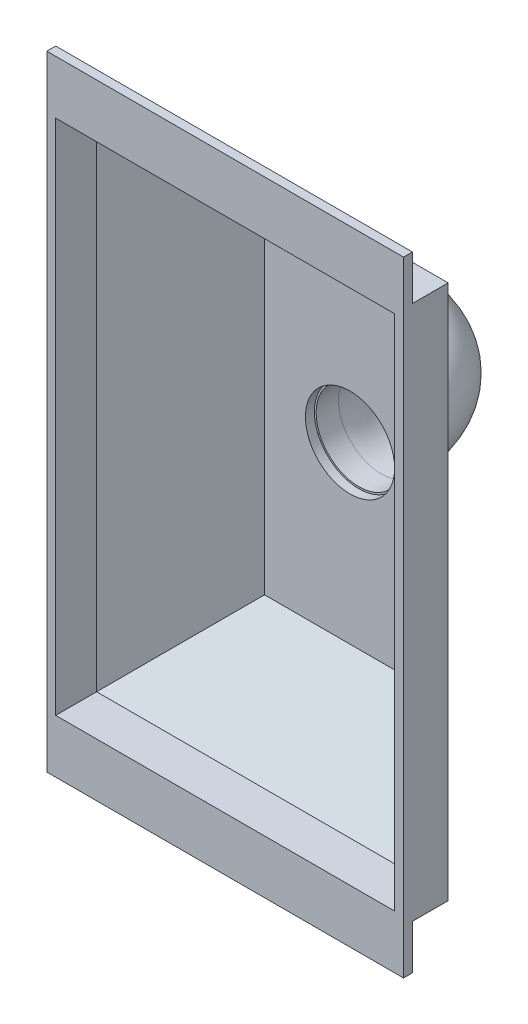
SolidWorks part; units mm, degrees
ref_plane "前视基准面" through (0, 0, 0) normal (0, 0, 1) x (1, 0, 0)
ref_plane "上视基准面" through (0, 0, 0) normal (0, 1, 0) x (1, 0, 0)
ref_plane "右视基准面" through (0, 0, 0) normal (1, 0, 0) x (0, 0, -1)
sketch "草图1" plane through (0, 0, 0) normal (0, 0, 1) x (1, 0, 0)
  line L1 (-200, -300) -> (200, -300)
  line L2 (-200, -300) -> (-200, 300)
  line L3 (-200, 300) -> (200, 300)
  line L4 (200, -300) -> (200, 300)
  line L5 (-200, -300) -> (200, 300) construction
  line L6 (-200, 300) -> (200, -300) construction
  point P0 (0, 0)
  dimension "D1" = 400
  dimension "D2" = 600
extrude "凸台-拉伸1" add sketch "草图1" along normal blind 150
sketch "草图2" plane through (0, -300, 0) normal (0, -1, 0) x (1, 0, 0)
  line L0 (0, 0) -> (0, 150) construction
  line L1 (-200, 150) -> (200, 150) construction
  line L2 (-200, 75) -> (-100, 0)
  line L3 (-200, 150) -> (-200, 0) construction
  line L4 (-200, 0) -> (200, 0) construction
  line L5 (-100, 0) -> (-200, 0)
  line L6 (-200, 0) -> (-200, 75)
  line L7 (200, 75) -> (100, 0)
  line L8 (200, 150) -> (200, 0) construction
  line L9 (100, 0) -> (200, 0)
  line L10 (200, 0) -> (200, 75)
  dimension "D1" = 200
  dimension "D2" = 100
extrude "切除-拉伸1" [suppressed] cut sketch "草图2" against normal through all
sketch "草图3" plane through (0, 0, 150) normal (0, 0, 1) x (1, 0, 0)
  line L0 (-200, -300) -> (200, -300) construction
  line L1 (-200, 300) -> (-260, 300)
  line L2 (-200, 300) -> (-200, -300)
  line L3 (-200, -300) -> (-260, -300)
  line L4 (-260, 300) -> (-260, -300)
  line L6 (200, 300) -> (260, 300)
  line L7 (200, 300) -> (200, -300)
  line L8 (200, -300) -> (260, -300)
  line L9 (260, 300) -> (260, -300)
  dimension "D1" = 60
extrude "凸台-拉伸2" [suppressed] add sketch "草图3" against normal blind 10
chamfer "倒角2" distance 100 angle 45 4 edges at (0, 300, 0) (-200, 0, 0) (0, -300, 0) (200, 0, 0)
shell "抽壳1" thickness 10
sketch "草图4" plane through (0, 0, 10) normal (0, 0, 1) x (1, 0, 0)
  circle A0 centre (0, 0) radius 50
  dimension "D1" = 100
extrude "切除-拉伸2" cut sketch "草图4" against normal through all
sketch "草图5" plane through (0, 0, 0) normal (0, 1, 0) x (1, 0, 0)
  line L0 (0, 0) -> (0, 25)
  line L1 (-100, 125) -> (-300, 125)
  arc A0 (0, 25) -> (-100, 125) centre (-100, 25) ccw
  point P6 (0, 125)
  dimension "D3" = 100
  dimension "D1" = 125
  dimension "D2" = 300
sketch "草图6" plane through (0, 0, 0) normal (0, 0, -1) x (-1, 0, 0)
  circle A0 centre (0, 0) radius 50
  dimension "D1" = 100
sweep "扫描1" add profiles "草图6" path "草图5"
shell "抽壳2" thickness 2
sketch "草图7" plane through (0, 0, 150) normal (0, 0, 1) x (1, 0, 0)
  line L0 (200, -300) -> (200, 300) construction
  line L1 (-200, 300) -> (200, 300)
  line L2 (-200, 300) -> (-200, 350)
  line L3 (-200, 350) -> (200, 350)
  line L4 (200, 300) -> (200, 350)
  line L6 (-200, -300) -> (200, -300)
  line L7 (-200, -300) -> (-200, -350)
  line L8 (-200, -350) -> (200, -350)
  line L9 (200, -300) -> (200, -350)
  dimension "D1" = 50
extrude "凸台-拉伸3" add sketch "草图7" against normal blind 10
